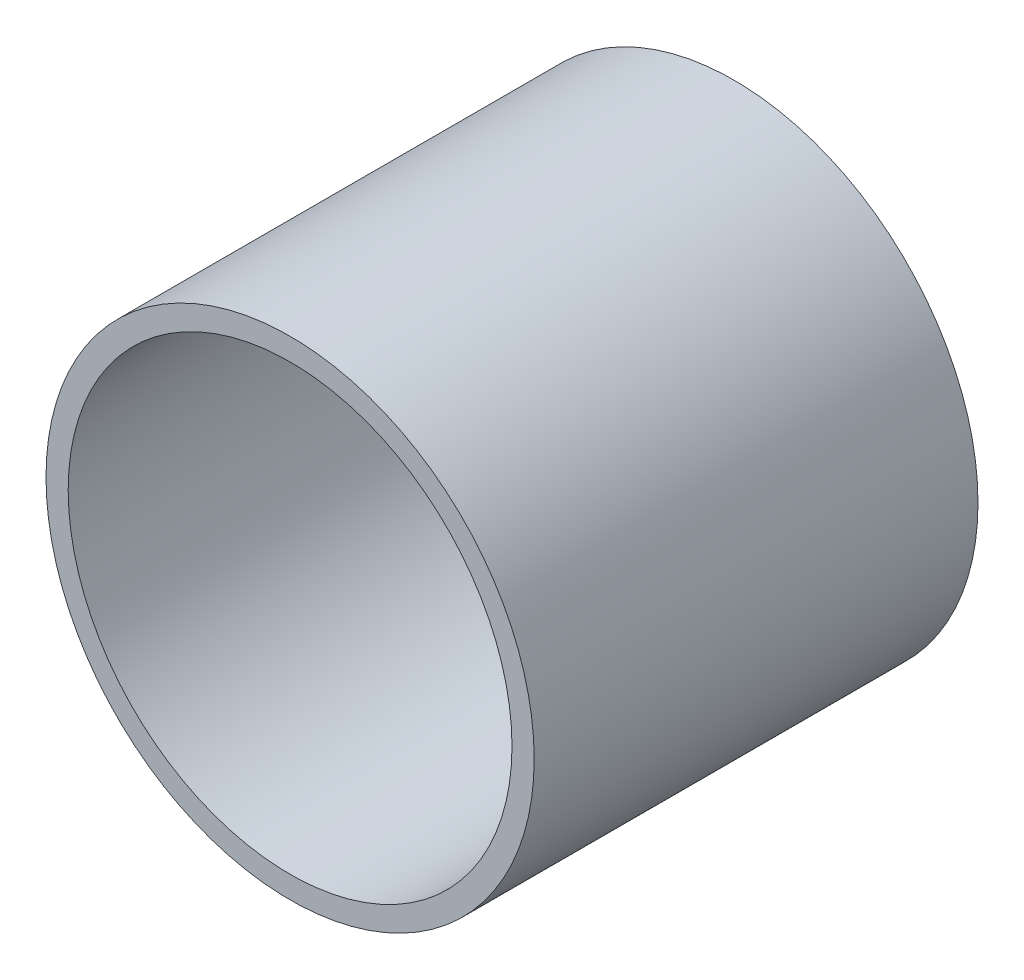
from build123d import *

# Parameters (mm, degrees)
SKETCH_1_R      = 110
SKETCH_1_R_2    = 100
EXTRUDE_1_DEPTH = 200


with BuildPart() as part:
    # 草图1 → 拉伸-薄壁1 (new body)
    with BuildSketch(Plane.XY):
        Circle(SKETCH_1_R)
        Circle(SKETCH_1_R_2, mode=Mode.SUBTRACT)
    extrude(amount=EXTRUDE_1_DEPTH)


solid = part.part
